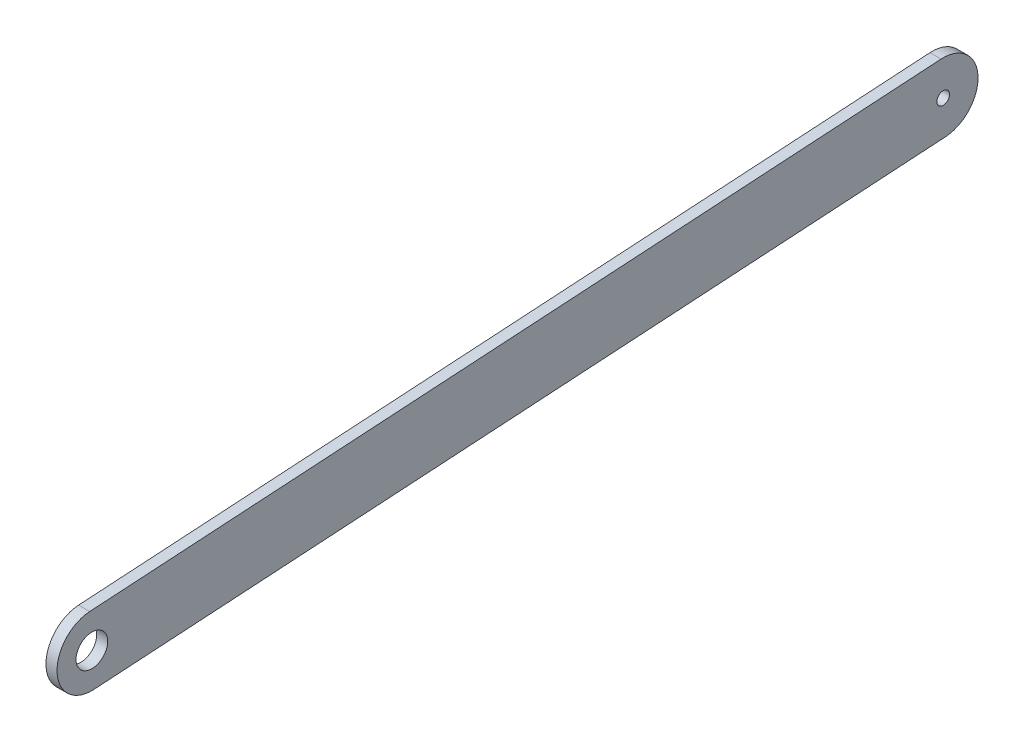
from build123d import *

# Parameters (mm, degrees)
SKETCH_1_R      = 4
SKETCH_1_R_2    = 10
EXTRUDE_1_DEPTH = 7


with BuildPart() as part:
    # 草图1 → 凸台-拉伸1 (new body)
    with BuildSketch(Plane(origin=(797.597549653, 0, 0), x_dir=(0, 0, -1), z_dir=(1, 0, 0))):
        with BuildLine():
            Line((-188.626135314, -11.329587329), (348.639550057, 21.957895527))
            ThreePointArc((348.639550057, 21.957895527), (371.957895527, 1.360449943), (351.360449943, -21.957895527))
            Line((351.360449943, -21.957895527), (-185.905235429, -55.245378382))
            ThreePointArc((-185.905235429, -55.245378382), (-209.223580898, -34.647932798), (-188.626135314, -11.329587329))
        make_face()
        with Locations(Location((350, 0, 0), (0, 0, 90))):
            Circle(SKETCH_1_R, mode=Mode.SUBTRACT)
        with Locations(Location((-187.265685371, -33.287482855, 0), (0, 0, 90))):
            Circle(SKETCH_1_R_2, mode=Mode.SUBTRACT)
    extrude(amount=-EXTRUDE_1_DEPTH)


solid = part.part
